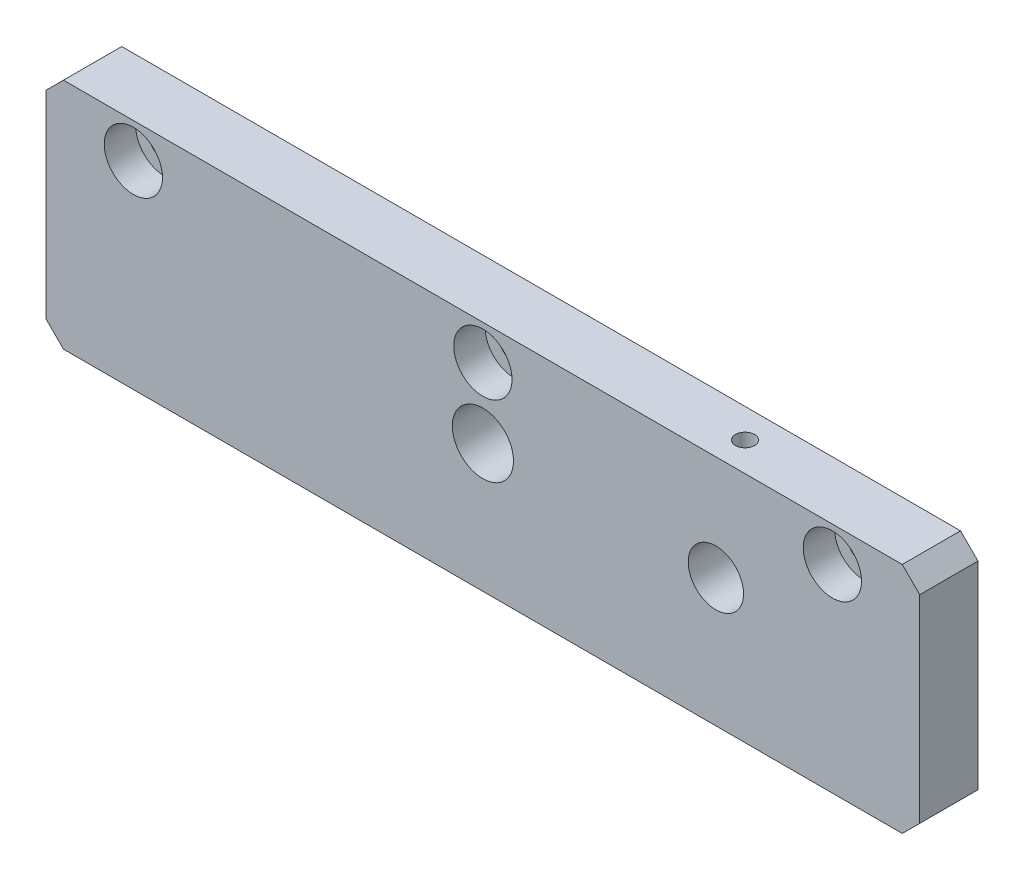
from build123d import *

# Parameters (mm, degrees)
SKETCH1_W                                           = 150
SKETCH1_H                                           = 40
BOSS_EXTRUDE1_DEPTH                                 = 10
SKETCH2_R                                           = 4.75
CUT_EXTRUDE1_DEPTH                                  = 79.262379212
F_10_5_10_5_DIAMETER_HOLE1_D                        = 10.5
F_10_5_10_5_DIAMETER_HOLE1_DEPTH                    = 76
F_10_5_10_5_DIAMETER_HOLE1_TIP                      = 3.15451825
CBORE_FOR_M5_HEX_SOCKET_HEAD_CAP_SCREW1_D           = 5.5
CBORE_FOR_M5_HEX_SOCKET_HEAD_CAP_SCREW1_CBORE_D     = 10
CBORE_FOR_M5_HEX_SOCKET_HEAD_CAP_SCREW1_CBORE_DEPTH = 5.4
M4_TAPPED_HOLE1_REACH                               = 87.586
M4_TAPPED_HOLE1_BORE_R                              = 1.65
CHAMFER1_SIZE                                       = 3


with BuildPart() as part:
    # Sketch1 → Boss-Extrude1 (new body)
    with BuildSketch(Plane.XY):
        Rectangle(SKETCH1_W, SKETCH1_H)
    extrude(amount=BOSS_EXTRUDE1_DEPTH)

    # Sketch2 → Cut-Extrude1 (cut, through all)
    with BuildSketch(Plane.XY.offset(10)):
        with Locations((40, 2)):
            Circle(SKETCH2_R)
    extrude(amount=-CUT_EXTRUDE1_DEPTH, mode=Mode.SUBTRACT)

    # Ø10.5 (10.5) Diameter Hole1
    with Locations(Plane.XY.offset(10)):
        with Locations((0, 2)):
            Hole(F_10_5_10_5_DIAMETER_HOLE1_D / 2, depth=F_10_5_10_5_DIAMETER_HOLE1_DEPTH)
            with Locations((0, 0, -(F_10_5_10_5_DIAMETER_HOLE1_DEPTH + F_10_5_10_5_DIAMETER_HOLE1_TIP / 2))):  # 118° drill point
                Cone(0, F_10_5_10_5_DIAMETER_HOLE1_D / 2, F_10_5_10_5_DIAMETER_HOLE1_TIP, mode=Mode.SUBTRACT)

    # CBORE for M5 Hex Socket Head Cap Screw1 (through all)
    with Locations(Plane.XY.offset(10)):
        with Locations((60, 14), (0, 14), (-60, 14)):
            CounterBoreHole(CBORE_FOR_M5_HEX_SOCKET_HEAD_CAP_SCREW1_D / 2, CBORE_FOR_M5_HEX_SOCKET_HEAD_CAP_SCREW1_CBORE_D / 2, CBORE_FOR_M5_HEX_SOCKET_HEAD_CAP_SCREW1_CBORE_DEPTH)

    # M4 Tapped Hole1 bore → M4 Tapped Hole1 (cut, up to next)
    with BuildSketch(Plane(origin=(0, 20, 0), x_dir=(1, 0, 0), z_dir=(0, 1, 0)), mode=Mode.PRIVATE) as m4_tapped_hole1_sk1:
        with Locations((40, -5)):
            Circle(M4_TAPPED_HOLE1_BORE_R)
    m4_tapped_hole1_tool1 = extrude(m4_tapped_hole1_sk1.sketch, amount=-M4_TAPPED_HOLE1_REACH, mode=Mode.PRIVATE) & part.part
    add(m4_tapped_hole1_tool1.solids().sort_by_distance((40, 20, 5))[0], mode=Mode.SUBTRACT)

    # Chamfer1
    chamfer1_edges = [part.edges().sort_by_distance(p)[0] for p in [
        (75, -20, 5),
        (-75, -20, 5),
        (-75, 20, 5),
        (75, 20, 5),
    ]]
    chamfer(chamfer1_edges, length=CHAMFER1_SIZE)


solid = part.part
